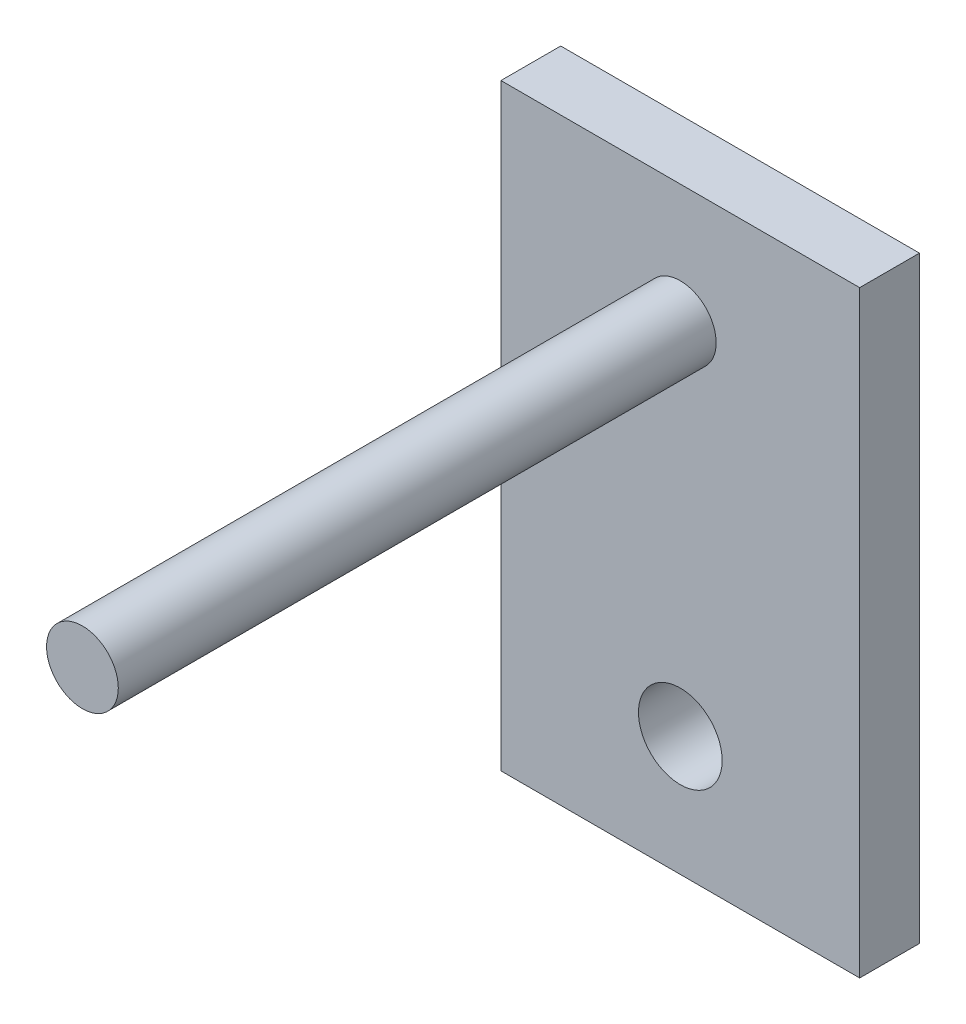
SolidWorks part; units mm, degrees
ref_plane "Front Plane" through (0, 0, 0) normal (0, 0, 1) x (1, 0, 0)
ref_plane "Top Plane" through (0, 0, 0) normal (0, 1, 0) x (1, 0, 0)
ref_plane "Right Plane" through (0, 0, 0) normal (1, 0, 0) x (0, 0, -1)
sketch "Sketch1" plane through (0, 0, 0) normal (0, 0, 1) x (1, 0, 0)
  line L0 (0, -30) -> (0, 0) construction
  line L1 (-30, -50) -> (30, -50)
  line L2 (-30, -50) -> (-30, 50)
  line L3 (-30, 50) -> (30, 50)
  line L4 (30, -50) -> (30, 50)
  line L5 (-30, -50) -> (30, 50) construction
  line L6 (-30, 50) -> (30, -50) construction
  circle A0 centre (0, -30) radius 7
  point P0 (0, 0)
  dimension "D3" = 14
  dimension "D4" = 20
  dimension "D1" = 60
  dimension "D2" = 100
extrude "Boss-Extrude1" add sketch "Sketch1" along normal blind 10
sketch "Sketch2" plane through (0, 0, 10) normal (0, 0, 1) x (1, 0, 0)
  line L0 (0, 0) -> (0, 50) construction
  line L1 (30, 50) -> (-30, 50) construction
  circle A0 centre (0, 30) radius 6
  dimension "D1" = 12
  dimension "D2" = 20
extrude "Boss-Extrude2" add sketch "Sketch2" along normal blind 100
